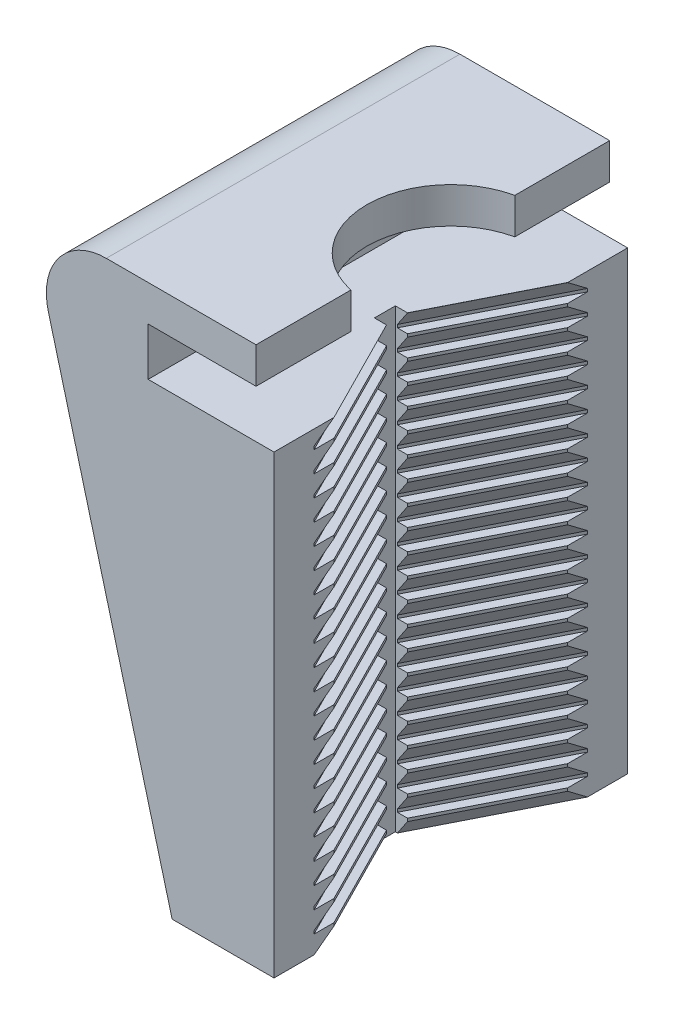
SolidWorks part; units mm, degrees
ref_plane "Front Plane" through (0, 0, 0) normal (0, 0, 1) x (1, 0, 0)
ref_plane "Top Plane" through (0, 0, 0) normal (0, 1, 0) x (1, 0, 0)
ref_plane "Right Plane" through (0, 0, 0) normal (1, 0, 0) x (0, 0, -1)
other "Configuration Table"
sketch "Sketch1" plane through (0, 0, 0) normal (0, 0, 1) x (1, 0, 0)
  line L0 (0, 0) -> (0, 76)
  line L1 (-3, 90) -> (-27.9839, 90)
  line L2 (-37.6462, 77.4234) -> (-17, 0)
  line L3 (-17, 0) -> (0, 0)
  line L7 (-3, 90) -> (-3, 84)
  line L8 (-3, 84) -> (-21, 84)
  line L9 (-21, 84) -> (-21, 76)
  line L10 (-21, 76) -> (0, 76)
  arc A0 (-27.9839, 90) -> (-37.6462, 77.4234) centre (-27.9839, 80) ccw
  point P15 (-41, 90)
  dimension "D13" = 10
  dimension "D2" = 90
  dimension "D3" = 17
  dimension "D8" = 6
  dimension "D9" = 8
  dimension "D10" = 21
  dimension "D11" = 3
  dimension "D12" = 41
extrude "Boss-Extrude1" add sketch "Sketch1" along normal blind 59
sketch "Sketch3" plane through (0, 90, 0) normal (0, 1, 0) x (1, 0, 0)
  line L0 (0, -59) -> (0, 0) construction
  circle A0 centre (0, -29.5) radius 14
  dimension "D1" = 28
extrude "Cut-Extrude2" cut sketch "Sketch3" against normal up to next
sketch "Sketch4" plane through (0, 0, 0) normal (0, -1, 0) x (-1, 0, 0)
  line L0 (0, -29.5) -> (17, -29.5) construction
  line L1 (0, -59) -> (0, 0) construction
  line L2 (17, -59) -> (17, 0) construction
  line L3 (9.3939, -30.4372) -> (0, -49)
  line L5 (11, -31.25) -> (11, -27.75)
  line L8 (11, -31.25) -> (-12.9526, -27.4394) construction
  line L9 (11, -27.75) -> (-11.9773, -31.4055) construction
  line L10 (17, -59) -> (0, -59) construction
  line L11 (11, -31.25) -> (9.3939, -30.4372)
  line L12 (11, -27.75) -> (9.3939, -28.5628)
  line L13 (9.3939, -28.5628) -> (0, -10)
  line L14 (0, -49) -> (0, -10)
  dimension "D1" = 3.5
  dimension "D2" = 6
  dimension "D3" = 10
  dimension "D4" = 1.8
extrude "Cut-Extrude3" cut sketch "Sketch4" against normal blind 80 and the other way through all
sketch "Sketch7" plane through (10.3474, 0, 20.4468) normal (-0.4515, 0, -0.8923) x (-0.8923, 0, 0.4515)
  line L0 (22.1253, 2.5) -> (23.6253, 0)
  line L1 (22.1253, 0) -> (22.1253, 76) construction
  line L2 (22.1253, 0) -> (23.9253, 0) construction
  line L3 (22.1253, 2.5) -> (22.1253, 3)
  line L4 (22.1253, 3) -> (23.6253, 3)
  line L5 (22.1253, 6) -> (23.6253, 3.5)
  line L6 (22.1253, 6) -> (22.1253, 6.5)
  line L7 (22.1253, 6.5) -> (23.6253, 6.5)
  line L8 (22.1253, 9.5) -> (23.6253, 7)
  line L9 (22.1253, 9.5) -> (22.1253, 10)
  line L10 (22.1253, 10) -> (23.6253, 10)
  line L11 (22.1253, 13) -> (23.6253, 10.5)
  line L12 (22.1253, 13) -> (22.1253, 13.5)
  line L13 (22.1253, 13.5) -> (23.6253, 13.5)
  line L14 (22.1253, 16.5) -> (23.6253, 14)
  line L15 (22.1253, 16.5) -> (22.1253, 17)
  line L16 (22.1253, 17) -> (23.6253, 17)
  line L17 (22.1253, 20) -> (23.6253, 17.5)
  line L18 (22.1253, 20) -> (22.1253, 20.5)
  line L19 (22.1253, 20.5) -> (23.6253, 20.5)
  line L20 (22.1253, 23.5) -> (23.6253, 21)
  line L21 (22.1253, 23.5) -> (22.1253, 24)
  line L22 (22.1253, 24) -> (23.6253, 24)
  line L23 (22.1253, 27) -> (23.6253, 24.5)
  line L24 (22.1253, 27) -> (22.1253, 27.5)
  line L25 (22.1253, 27.5) -> (23.6253, 27.5)
  line L26 (22.1253, 30.5) -> (23.6253, 28)
  line L27 (22.1253, 30.5) -> (22.1253, 31)
  line L28 (22.1253, 31) -> (23.6253, 31)
  line L29 (22.1253, 34) -> (23.6253, 31.5)
  line L30 (22.1253, 34) -> (22.1253, 34.5)
  line L31 (22.1253, 34.5) -> (23.6253, 34.5)
  line L32 (22.1253, 37.5) -> (23.6253, 35)
  line L33 (22.1253, 37.5) -> (22.1253, 38)
  line L34 (22.1253, 38) -> (23.6253, 38)
  line L35 (22.1253, 41) -> (23.6253, 38.5)
  line L36 (22.1253, 41) -> (22.1253, 41.5)
  line L37 (22.1253, 41.5) -> (23.6253, 41.5)
  line L38 (22.1253, 44.5) -> (23.6253, 42)
  line L39 (22.1253, 44.5) -> (22.1253, 45)
  line L40 (22.1253, 45) -> (23.6253, 45)
  line L41 (22.1253, 48) -> (23.6253, 45.5)
  line L42 (22.1253, 48) -> (22.1253, 48.5)
  line L43 (22.1253, 48.5) -> (23.6253, 48.5)
  line L44 (22.1253, 51.5) -> (23.6253, 49)
  line L45 (22.1253, 51.5) -> (22.1253, 52)
  line L46 (22.1253, 52) -> (23.6253, 52)
  line L47 (22.1253, 55) -> (23.6253, 52.5)
  line L48 (22.1253, 55) -> (22.1253, 55.5)
  line L49 (22.1253, 55.5) -> (23.6253, 55.5)
  line L50 (22.1253, 58.5) -> (23.6253, 56)
  line L51 (22.1253, 58.5) -> (22.1253, 59)
  line L52 (22.1253, 59) -> (23.6253, 59)
  line L53 (22.1253, 62) -> (23.6253, 59.5)
  line L54 (22.1253, 62) -> (22.1253, 62.5)
  line L55 (22.1253, 62.5) -> (23.6253, 62.5)
  line L56 (22.1253, 65.5) -> (23.6253, 63)
  line L57 (22.1253, 65.5) -> (22.1253, 66)
  line L58 (22.1253, 66) -> (23.6253, 66)
  line L59 (22.1253, 69) -> (23.6253, 66.5)
  line L60 (22.1253, 69) -> (22.1253, 69.5)
  line L61 (22.1253, 69.5) -> (23.6253, 69.5)
  line L62 (22.1253, 72.5) -> (23.6253, 70)
  line L63 (22.1253, 72.5) -> (22.1253, 73)
  line L64 (22.1253, 73) -> (23.6253, 73)
  line L65 (22.1253, 76) -> (23.6253, 73.5)
  line L66 (22.1253, 76) -> (22.1253, 76.5)
  line L68 (23.6253, 3) -> (23.6253, 3.5)
  line L70 (23.6253, 73) -> (23.6253, 73.5)
  line L71 (23.6253, 69.5) -> (23.6253, 70)
  line L72 (23.6253, 66) -> (23.6253, 66.5)
  line L73 (23.6253, 62.5) -> (23.6253, 63)
  line L74 (23.6253, 59) -> (23.6253, 59.5)
  line L75 (23.6253, 55.5) -> (23.6253, 56)
  line L76 (23.6253, 52) -> (23.6253, 52.5)
  line L77 (23.6253, 48.5) -> (23.6253, 49)
  line L78 (23.6253, 45) -> (23.6253, 45.5)
  line L79 (23.6253, 41.5) -> (23.6253, 42)
  line L80 (23.6253, 38) -> (23.6253, 38.5)
  line L81 (23.6253, 34.5) -> (23.6253, 35)
  line L82 (23.6253, 31) -> (23.6253, 31.5)
  line L83 (23.6253, 27.5) -> (23.6253, 28)
  line L84 (23.6253, 24) -> (23.6253, 24.5)
  line L85 (23.6253, 20.5) -> (23.6253, 21)
  line L86 (23.6253, 17) -> (23.6253, 17.5)
  line L87 (23.6253, 13.5) -> (23.6253, 14)
  line L88 (23.6253, 10) -> (23.6253, 10.5)
  line L89 (23.6253, 6.5) -> (23.6253, 7)
  line L90 (23.6253, 0) -> (21.0866, -2.1997)
  line L91 (21.0866, -2.1997) -> (20.0439, 77.69)
  line L92 (20.0439, 77.69) -> (22.1253, 76.5)
  line L94 (22.1253, 76.5) -> (23.6253, 76.5) [skipped]
  dimension "D1" = 1.5
  dimension "D3" = 0.5
  dimension "D5" = 22
extrude "Cut-Extrude5" cut sketch "Sketch7" against normal blind 80
sketch "Sketch8" plane through (-13.4228, 0, 26.5239) normal (-0.4515, 0, 0.8923) x (0.8923, 0, 0.4515)
  line L89 (4.5154, 0) -> (4.5154, 110.1549) construction
  line L91 (6.5968, 77.672) -> (4.5154, 76.482)
  line L92 (5.5541, -2.2177) -> (6.5968, 77.672)
  line L93 (3.0154, -0.018) -> (5.5541, -2.2177)
  line L94 (3.0154, 6.482) -> (3.0154, 6.982)
  line L95 (3.0154, 9.982) -> (3.0154, 10.482)
  line L96 (3.0154, 13.482) -> (3.0154, 13.982)
  line L97 (3.0154, 16.982) -> (3.0154, 17.482)
  line L98 (3.0154, 20.482) -> (3.0154, 20.982)
  line L99 (3.0154, 23.982) -> (3.0154, 24.482)
  line L100 (3.0154, 27.482) -> (3.0154, 27.982)
  line L101 (3.0154, 30.982) -> (3.0154, 31.482)
  line L102 (3.0154, 34.482) -> (3.0154, 34.982)
  line L103 (3.0154, 37.982) -> (3.0154, 38.482)
  line L104 (3.0154, 41.482) -> (3.0154, 41.982)
  line L105 (3.0154, 44.982) -> (3.0154, 45.482)
  line L106 (3.0154, 48.482) -> (3.0154, 48.982)
  line L107 (3.0154, 51.982) -> (3.0154, 52.482)
  line L108 (3.0154, 55.482) -> (3.0154, 55.982)
  line L109 (3.0154, 58.982) -> (3.0154, 59.482)
  line L110 (3.0154, 62.482) -> (3.0154, 62.982)
  line L111 (3.0154, 65.982) -> (3.0154, 66.482)
  line L112 (3.0154, 69.482) -> (3.0154, 69.982)
  line L113 (3.0154, 72.982) -> (3.0154, 73.482)
  line L114 (3.0154, 2.982) -> (3.0154, 3.482)
  line L115 (4.5154, 75.982) -> (4.5154, 76.482)
  line L116 (4.5154, 75.982) -> (3.0154, 73.482)
  line L117 (4.5154, 72.982) -> (3.0154, 72.982)
  line L118 (4.5154, 72.482) -> (4.5154, 72.982)
  line L119 (4.5154, 72.482) -> (3.0154, 69.982)
  line L120 (4.5154, 69.482) -> (3.0154, 69.482)
  line L121 (4.5154, 68.982) -> (4.5154, 69.482)
  line L122 (4.5154, 68.982) -> (3.0154, 66.482)
  line L123 (4.5154, 65.982) -> (3.0154, 65.982)
  line L124 (4.5154, 65.482) -> (4.5154, 65.982)
  line L125 (4.5154, 65.482) -> (3.0154, 62.982)
  line L126 (4.5154, 62.482) -> (3.0154, 62.482)
  line L127 (4.5154, 61.982) -> (4.5154, 62.482)
  line L128 (4.5154, 61.982) -> (3.0154, 59.482)
  line L129 (4.5154, 58.982) -> (3.0154, 58.982)
  line L130 (4.5154, 58.482) -> (4.5154, 58.982)
  line L131 (4.5154, 58.482) -> (3.0154, 55.982)
  line L132 (4.5154, 55.482) -> (3.0154, 55.482)
  line L133 (4.5154, 54.982) -> (4.5154, 55.482)
  line L134 (4.5154, 54.982) -> (3.0154, 52.482)
  line L135 (4.5154, 51.982) -> (3.0154, 51.982)
  line L136 (4.5154, 51.482) -> (4.5154, 51.982)
  line L137 (4.5154, 51.482) -> (3.0154, 48.982)
  line L138 (4.5154, 48.482) -> (3.0154, 48.482)
  line L139 (4.5154, 47.982) -> (4.5154, 48.482)
  line L140 (4.5154, 47.982) -> (3.0154, 45.482)
  line L141 (4.5154, 44.982) -> (3.0154, 44.982)
  line L142 (4.5154, 44.482) -> (4.5154, 44.982)
  line L143 (4.5154, 44.482) -> (3.0154, 41.982)
  line L144 (4.5154, 41.482) -> (3.0154, 41.482)
  line L145 (4.5154, 40.982) -> (4.5154, 41.482)
  line L146 (4.5154, 40.982) -> (3.0154, 38.482)
  line L147 (4.5154, 37.982) -> (3.0154, 37.982)
  line L148 (4.5154, 37.482) -> (4.5154, 37.982)
  line L149 (4.5154, 37.482) -> (3.0154, 34.982)
  line L150 (4.5154, 34.482) -> (3.0154, 34.482)
  line L151 (4.5154, 33.982) -> (4.5154, 34.482)
  line L152 (4.5154, 33.982) -> (3.0154, 31.482)
  line L153 (4.5154, 30.982) -> (3.0154, 30.982)
  line L154 (4.5154, 30.482) -> (4.5154, 30.982)
  line L155 (4.5154, 30.482) -> (3.0154, 27.982)
  line L156 (4.5154, 27.482) -> (3.0154, 27.482)
  line L157 (4.5154, 26.982) -> (4.5154, 27.482)
  line L158 (4.5154, 26.982) -> (3.0154, 24.482)
  line L159 (4.5154, 23.982) -> (3.0154, 23.982)
  line L160 (4.5154, 23.482) -> (4.5154, 23.982)
  line L161 (4.5154, 23.482) -> (3.0154, 20.982)
  line L162 (4.5154, 20.482) -> (3.0154, 20.482)
  line L163 (4.5154, 19.982) -> (4.5154, 20.482)
  line L164 (4.5154, 19.982) -> (3.0154, 17.482)
  line L165 (4.5154, 16.982) -> (3.0154, 16.982)
  line L166 (4.5154, 16.482) -> (4.5154, 16.982)
  line L167 (4.5154, 16.482) -> (3.0154, 13.982)
  line L168 (4.5154, 13.482) -> (3.0154, 13.482)
  line L169 (4.5154, 12.982) -> (4.5154, 13.482)
  line L170 (4.5154, 12.982) -> (3.0154, 10.482)
  line L171 (4.5154, 9.982) -> (3.0154, 9.982)
  line L172 (4.5154, 9.482) -> (4.5154, 9.982)
  line L173 (4.5154, 9.482) -> (3.0154, 6.982)
  line L174 (4.5154, 6.482) -> (3.0154, 6.482)
  line L175 (4.5154, 5.982) -> (4.5154, 6.482)
  line L176 (4.5154, 5.982) -> (3.0154, 3.482)
  line L177 (4.5154, 2.982) -> (3.0154, 2.982)
  line L178 (4.5154, 2.482) -> (4.5154, 2.982)
  line L179 (4.5154, 2.482) -> (3.0154, -0.018)
extrude "Cut-Extrude6" cut sketch "Sketch8" against normal through all
sketch "Sketch9" plane through (0, 0, 0) normal (0, -1, 0) x (-1, 0, 0)
  line L1 (11, -31.25) -> (7.8762, -31.25)
  line L2 (11, -31.25) -> (11, -27.75)
  line L3 (11, -27.75) -> (7.8762, -27.75)
  line L4 (7.8762, -31.25) -> (7.8762, -27.75)
extrude "Cut-Extrude7" cut sketch "Sketch9" against normal blind 80
